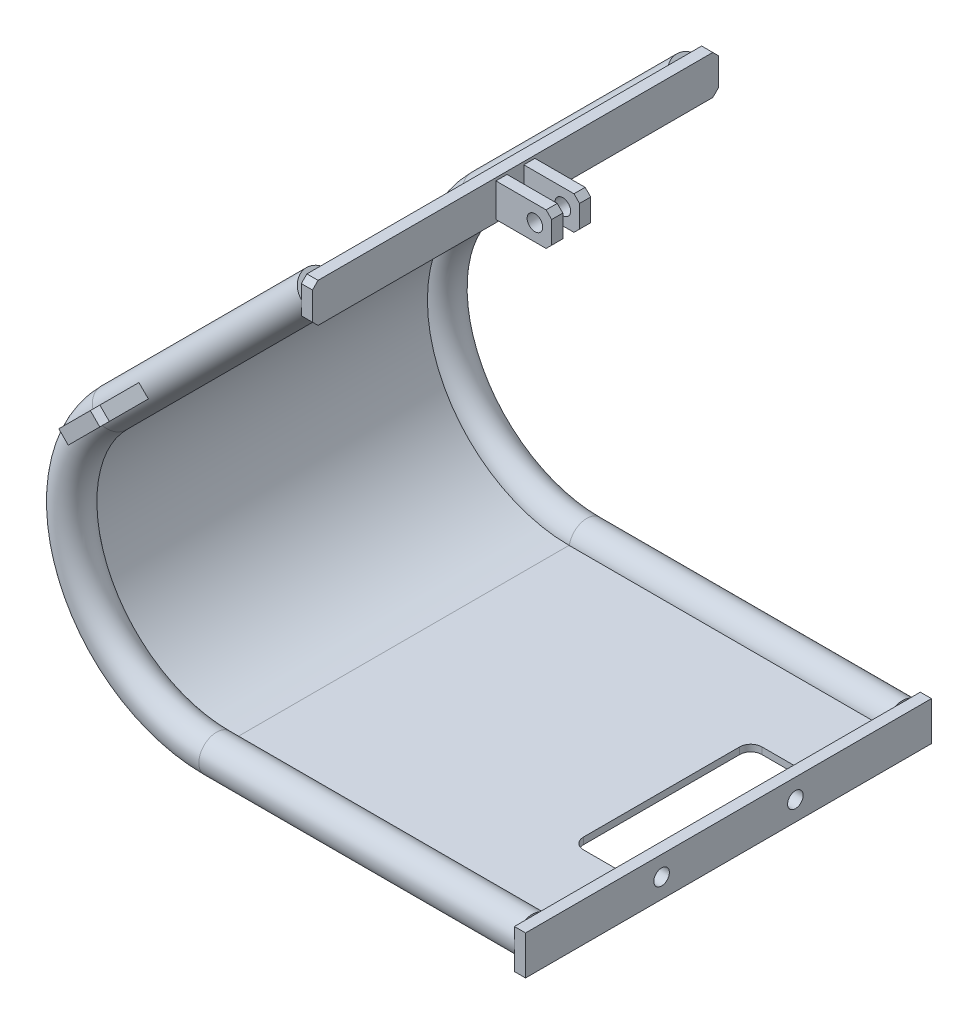
SolidWorks part; units mm, degrees
material "Q235-A "
ref_plane "前视基准面" through (0, 0, 0) normal (0, 0, 1) x (1, 0, 0)
ref_plane "上视基准面" through (0, 0, 0) normal (0, 1, 0) x (1, 0, 0)
ref_plane "右视基准面" through (0, 0, 0) normal (1, 0, 0) x (0, 0, -1)
sketch "草图1" plane through (0, 0, 0) normal (0, 0, 1) x (1, 0, 0)
  line L0 (0, 0) -> (-183.8478, -183.8478)
  line L1 (-91.9239, -405.7716) -> (191.0761, -405.7716)
  arc A0 (-183.8478, -183.8478) -> (-91.9239, -405.7716) centre (-91.9239, -275.7716) ccw
  dimension "D1" = 130
  dimension "D2" = 260
  dimension "D3" = 283
  dimension "D4" = 45
ref_plane "基准面1" through (191.0761, 0, 0) normal (1, 0, 0) x (0, 0, -1)
sketch "草图2" plane through (191.0761, 0, 0) normal (1, 0, 0) x (0, 0, -1)
  line L0 (0, 242.55) -> (0, -242.55) construction
  line L1 (0, -183.8478) -> (0, -405.7716) construction
  circle A0 centre (0, -405.7716) radius 16
  circle A1 centre (0, -405.7716) radius 11
  dimension "D1" = 32
  dimension "D2" = 5
sweep "扫描1" add profiles "草图2" path "草图1"
sketch "草图4" plane through (0, 0, 0) normal (0, 0, 1) x (1, 0, 0)
  line L0 (0, 0) -> (0, -67.9333)
  line L1 (0, -17.6) -> (0, 17.6) construction
  line L2 (0, -67.9333) -> (55.6423, -67.9333)
  line L3 (55.6423, -67.9333) -> (55.6423, 0)
  line L4 (17.6, 0) -> (-17.6, 0) construction
  line L5 (55.6423, 0) -> (0, 0)
extrude "切除-拉伸1" cut sketch "草图4" against normal through all both and the other way through all
sketch "草图6" plane through (0, 0, 0) normal (0, 0, 1) x (1, 0, 0)
  line L0 (-91.9239, -405.7716) -> (191.0761, -405.7716) construction
  line L1 (0, 0) -> (-183.8478, -183.8478) construction
  line L2 (-91.9239, -405.7716) -> (191.0761, -405.7716)
  line L3 (0, 0) -> (-183.8478, -183.8478)
  arc A0 (-183.8478, -183.8478) -> (-91.9239, -405.7716) centre (-91.9239, -275.7716) ccw construction
  arc A1 (-183.8478, -183.8478) -> (-91.9239, -405.7716) centre (-91.9239, -275.7716) ccw
extrude "拉伸-薄壁2" add sketch "草图6" along normal blind 300 from offset 16 thin thin type mid plane wall 6
ref_plane "基准面3" through (0, 0, 166) normal (0, 0, 1) x (1, 0, 0)
sketch "草图7" plane through (191.0761, 0, 0) normal (1, 0, 0) x (0, 0, -1)
  line L0 (-166, -408.7716) -> (-166, -435.7957) construction
  line L1 (-316, -408.7716) -> (-16, -408.7716) construction
  circle A0 centre (0, -405.7716) radius 16 construction
  circle A1 centre (0, -405.7716) radius 11 construction
  circle A2 centre (0, -405.7716) radius 16 construction
  circle A3 centre (0, -405.7716) radius 11 construction
  circle A4 centre (-332, -405.7716) radius 11
  circle A5 centre (-332, -405.7716) radius 16
ref_plane "基准面4" through (0, 0, 332) normal (0, 0, 1) x (1, 0, 0)
sketch "草图8" plane through (0, 0, 332) normal (0, 0, 1) x (1, 0, 0)
  line L0 (0, 0) -> (-183.8478, -183.8478) construction
  line L1 (-91.9239, -405.7716) -> (191.0761, -405.7716) construction
  line L2 (0, 0) -> (-183.8478, -183.8478)
  line L3 (-91.9239, -405.7716) -> (191.0761, -405.7716)
  arc A0 (-183.8478, -183.8478) -> (-91.9239, -405.7716) centre (-91.9239, -275.7716) ccw construction
  arc A1 (-183.8478, -183.8478) -> (-91.9239, -405.7716) centre (-91.9239, -275.7716) ccw
sweep "扫描2" add profiles "草图7" path "草图8"
sketch "草图9" plane through (0, 0, 0) normal (1, 0, 0) x (0, 0, -1)
  line L0 (-316, -2.1213) -> (-16, -2.1213) construction
  line L1 (-422.7489, 37.0269) -> (90.7489, 37.0269)
  line L2 (-422.7489, 37.0269) -> (-422.7489, -41.2696)
  line L3 (-422.7489, -41.2696) -> (90.7489, -41.2696)
  line L4 (90.7489, 37.0269) -> (90.7489, -41.2696)
  line L5 (-422.7489, 37.0269) -> (90.7489, -41.2696) construction
  line L6 (-422.7489, -41.2696) -> (90.7489, 37.0269) construction
  point P0 (-166, -2.1213)
extrude "切除-拉伸2" cut sketch "草图9" along normal through all
sketch "草图10" plane through (0, 0, 0) normal (1, 0, 0) x (0, 0, -1)
  line L0 (-316, 0) -> (-16, 0) construction
  line L1 (-348, 17.5) -> (16, 17.5)
  line L2 (-348, 17.5) -> (-348, -17.5)
  line L3 (-348, -17.5) -> (16, -17.5)
  line L4 (16, 17.5) -> (16, -17.5)
  line L5 (-348, 17.5) -> (16, -17.5) construction
  line L6 (-348, -17.5) -> (16, 17.5) construction
  line L7 (16, -183.8478) -> (16, 0) construction
  point P0 (-166, 0)
  dimension "D1" = 35
extrude "凸台-拉伸2" add sketch "草图10" along normal blind 10 separate body
sketch "草图11" plane through (191.0761, 0, 0) normal (1, 0, 0) x (0, 0, -1)
  line L0 (16, -405.7716) -> (16, -183.8478) construction
  line L1 (-348, -391.2716) -> (16, -391.2716)
  line L2 (-348, -391.2716) -> (-348, -426.2716)
  line L3 (-348, -426.2716) -> (16, -426.2716)
  line L4 (16, -391.2716) -> (16, -426.2716)
  line L5 (-348, -391.2716) -> (16, -426.2716) construction
  line L6 (-348, -426.2716) -> (16, -391.2716) construction
  point P0 (-166, -408.7716)
  dimension "D1" = 35
extrude "凸台-拉伸4" add sketch "草图11" along normal blind 10 separate body
chamfer "倒角1" distance 5 angle 45 4 edges at (5, 17.5, -16) (5, -17.5, -16) (5, -17.5, 348) (5, 17.5, 348)
sketch "草图13" plane through (0, -402.7716, 0) normal (0, 1, 0) x (1, 0, 0)
  line L0 (191.0761, -166) -> (166.0761, -166) construction
  line L1 (191.0761, 16) -> (191.0761, -348) construction
  line L2 (191.0761, -316) -> (191.0761, -16) construction
  line L3 (151.0761, -246) -> (191.0761, -246)
  line L4 (141.0761, -236) -> (141.0761, -96)
  line L5 (151.0761, -86) -> (191.0761, -86)
  line L6 (191.0761, -246) -> (191.0761, -86)
  line L7 (141.0761, -246) -> (191.0761, -86) construction
  line L8 (141.0761, -86) -> (191.0761, -246) construction
  arc A0 (151.0761, -246) -> (141.0761, -236) centre (151.0761, -236) cw
  arc A1 (141.0761, -96) -> (151.0761, -86) centre (151.0761, -96) cw
  dimension "D3" = 10
  dimension "D1" = 160
  dimension "D2" = 50
extrude "切除-拉伸4" cut sketch "草图13" against normal through all
sketch "草图14" plane through (201.0761, 0, 0) normal (1, 0, 0) x (0, 0, -1)
  line L0 (-166, -391.2716) -> (-166, -408.7716) construction
  line L1 (16, -391.2716) -> (-348, -391.2716) construction
  line L2 (-166, -408.7716) -> (16, -408.7716) construction
  line L3 (16, -426.2716) -> (16, -391.2716) construction
  circle A0 centre (-106, -408.7716) radius 7
  circle A1 centre (-226, -408.7716) radius 7
  dimension "D1" = 14
  dimension "D2" = 120
extrude "切除-拉伸5" cut sketch "草图14" against normal up to next (10 mm away)
sketch "草图15" plane through (10, 0, 0) normal (1, 0, 0) x (0, 0, -1)
  line L0 (-166, 17.5) -> (-166, -17.5) construction
  line L1 (11, 17.5) -> (-343, 17.5) construction
  line L2 (-343, -17.5) -> (11, -17.5) construction
  line L3 (-166, 0) -> (-178.5, 0) construction
  line L8 (-148.5, -15) -> (-158.5, 15) construction
  line L9 (-183.5, 15) -> (-173.5, 15)
  line L10 (-183.5, 15) -> (-183.5, -15)
  line L11 (-183.5, -15) -> (-173.5, -15)
  line L12 (-173.5, 15) -> (-173.5, -15)
  line L13 (-183.5, 15) -> (-173.5, -15) construction
  line L14 (-183.5, -15) -> (-173.5, 15) construction
  line L15 (-148.5, 15) -> (-158.5, -15) construction
  line L16 (-158.5, 15) -> (-158.5, -15)
  line L17 (-148.5, -15) -> (-158.5, -15)
  line L18 (-148.5, 15) -> (-148.5, -15)
  line L19 (-148.5, 15) -> (-158.5, 15)
  dimension "D1" = 10
  dimension "D2" = 30
  dimension "D3" = 7.5
extrude "凸台-拉伸5" add sketch "草图15" along normal blind 50 separate body
chamfer "倒角2" distance 5 angle 45 2 edges at (60, -15, 178.5) (60, 15, 178.5)
chamfer "倒角3" distance 5 angle 45 2 edges at (60, -15, 153.5) (60, 15, 153.5)
sketch "草图16" plane through (0, 0, 183.5) normal (0, 0, 1) x (1, 0, 0)
  line L0 (60, 0) -> (45, 0) construction
  line L1 (60, 10) -> (60, -10) construction
  circle A0 centre (45, 0) radius 7
  dimension "D1" = 14
  dimension "D2" = 15
extrude "切除-拉伸6" cut sketch "草图16" against normal through all
ref_plane "基准面5" through (0, 0, 0) normal (-0.7071, 0.7071, 0) x (0.7071, 0.7071, 0)
sketch "草图18" plane through (0, 0, 0) normal (-0.7071, 0.7071, 0) x (0.7071, 0.7071, 0)
  line L0 (0, 16) -> (-260, 16) construction
  line L1 (-250, 16) -> (-200, 16)
  line L2 (-250, 16) -> (-250, 56)
  line L3 (-250, 56) -> (-200, 56)
  line L4 (-200, 16) -> (-200, 56)
  line L5 (0, -16) -> (0, 16) construction
  line L6 (-225, 56) -> (-225, 41) construction
  line L7 (19.4454, -166) -> (-441.1386, -166) construction
  line L8 (19.4454, 11) -> (19.4454, -343) construction
  line L9 (-225, -388) -> (-225, -373) construction
  line L10 (-200, -348) -> (-200, -388)
  line L11 (-250, -388) -> (-200, -388)
  line L12 (-250, -348) -> (-250, -388)
  line L13 (-250, -348) -> (-200, -348)
  circle A0 centre (-225, 41) radius 7
  circle A1 centre (-225, -373) radius 7
  dimension "D4" = 14
  dimension "D1" = 50
  dimension "D2" = 40
  dimension "D3" = 200
  dimension "D5" = 15
extrude "凸台-拉伸6" add sketch "草图18" along normal mid plane 12
chamfer "倒角4" distance 5 angle 45 2 edges at (-141.4214, -141.4214, -56) (-176.7767, -176.7767, -56)
ref_plane "基准面6" through (0, 0, 166) normal (0, 0, 1) x (1, 0, 0)
chamfer "倒角5" distance 5 angle 45 2 edges at (-141.4214, -141.4214, 388) (-176.7767, -176.7767, 388)
